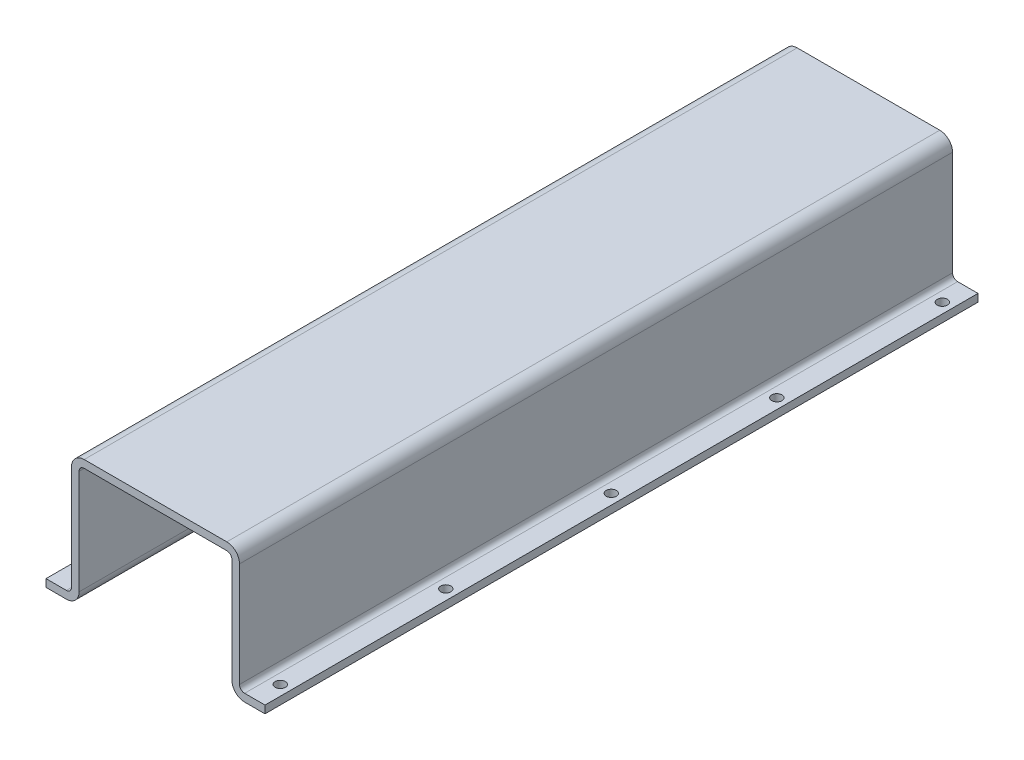
SolidWorks part; units mm, degrees
ref_plane "Front Plane" through (0, 0, 0) normal (0, 0, 1) x (1, 0, 0)
ref_plane "Top Plane" through (0, 0, 0) normal (0, 1, 0) x (1, 0, 0)
ref_plane "Right Plane" through (0, 0, 0) normal (1, 0, 0) x (0, 0, -1)
sketch "Sketch1" plane through (0, 0, 0) normal (0, 0, 1) x (1, 0, 0)
  line L1 (86, 0) -> (86, 3)
  line L2 (86, 3) -> (78, 3)
  line L3 (76, 5) -> (76, 46)
  line L4 (71, 51) -> (15, 51)
  line L5 (10, 46) -> (10, 5)
  line L6 (8, 3) -> (0, 3)
  line L7 (0, 3) -> (0, 0)
  line L8 (86, 0) -> (78, 0)
  line L9 (73, 5) -> (73, 46)
  line L10 (71, 48) -> (15, 48)
  line L11 (13, 46) -> (13, 5)
  line L12 (8, 0) -> (0, 0)
  arc A0 (78, 3) -> (76, 5) centre (78, 5) cw
  arc A1 (10, 5) -> (8, 3) centre (8, 5) cw
  arc A2 (76, 46) -> (71, 51) centre (71, 46) ccw
  arc A3 (15, 51) -> (10, 46) centre (15, 46) ccw
  arc A4 (78, 0) -> (73, 5) centre (78, 5) cw
  arc A5 (73, 46) -> (71, 48) centre (71, 46) ccw
  arc A6 (15, 48) -> (13, 46) centre (15, 46) ccw
  arc A7 (13, 5) -> (8, 0) centre (8, 5) cw
  point P11 (76, 3)
  point P14 (10, 3)
  point P17 (76, 51)
  point P20 (10, 51)
  dimension "D7" = 2
  dimension "D8" = 5
  dimension "D1" = 66
  dimension "D2" = 10
  dimension "D3" = 10
  dimension "D4" = 48
  dimension "D5" = 48
  dimension "D6" = 3
extrude "Boss-Extrude1" add sketch "Sketch1" along normal blind 280
sketch "Sketch7" plane through (0, 0, 0) normal (0, -1, 0) x (-1, 0, 0)
  line L0 (-78, -280) -> (-86, -280) construction
  line L1 (-86, -280) -> (-86, 0) construction
  line L2 (0, -280) -> (-8, -280) construction
  line L3 (0, -280) -> (0, 0) construction
  circle A0 centre (-4, -270) radius 2
  circle A1 centre (-82, -270) radius 2
  dimension "D1" = 10
  dimension "D2" = 4
  dimension "D3" = 4
  dimension "D4" = 4
  dimension "D5" = 10
  dimension "D6" = 4
extrude "Cut-Extrude3" cut sketch "Sketch7" against normal blind 10
pattern_linear "LPattern1" count 5 spacing 65 along (0, 0, -1) of "Cut-Extrude3"
